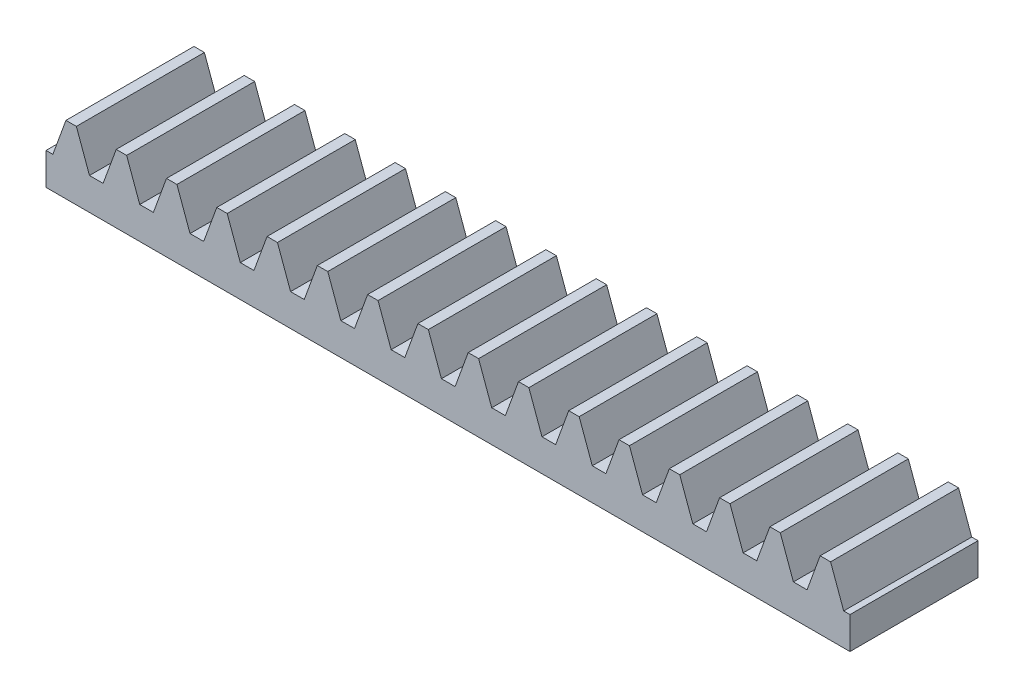
SolidWorks part; units mm, degrees
ref_plane "Front Plane" through (0, 0, 0) normal (0, 0, 1) x (1, 0, 0)
ref_plane "Top Plane" through (0, 0, 0) normal (0, 1, 0) x (1, 0, 0)
ref_plane "Right Plane" through (0, 0, 0) normal (1, 0, 0) x (0, 0, -1)
other "Configuration Table"
sketch "Sketch1" plane through (0, 0, 0) normal (0, 0, 1) x (1, 0, 0)
  line L0 (7.8146, 19.5625) -> (7.6014, 19.5625)
  line L1 (7.6014, 19.5625) -> (7.3966, 20.125)
  line L2 (7.3966, 20.125) -> (7.2339, 20.125)
  line L3 (7.2339, 20.125) -> (7.0292, 19.5625)
  line L4 (7.0292, 19.5625) -> (6.816, 19.5625)
  line L5 (6.816, 19.5625) -> (6.6112, 20.125)
  line L6 (6.6112, 20.125) -> (6.4485, 20.125)
  line L7 (6.4485, 20.125) -> (6.2438, 19.5625)
  line L8 (6.2438, 19.5625) -> (6.0306, 19.5625)
  line L9 (6.0306, 19.5625) -> (5.8258, 20.125)
  line L10 (5.8258, 20.125) -> (5.6631, 20.125)
  line L11 (5.6631, 20.125) -> (5.4584, 19.5625)
  line L12 (5.4584, 19.5625) -> (5.2452, 19.5625)
  line L13 (5.2452, 19.5625) -> (5.0404, 20.125)
  line L14 (5.0404, 20.125) -> (4.8777, 20.125)
  line L15 (4.8777, 20.125) -> (4.673, 19.5625)
  line L16 (4.673, 19.5625) -> (4.4598, 19.5625)
  line L17 (4.4598, 19.5625) -> (4.255, 20.125)
  line L18 (4.255, 20.125) -> (4.0923, 20.125)
  line L19 (4.0923, 20.125) -> (3.8876, 19.5625)
  line L20 (3.8876, 19.5625) -> (3.6744, 19.5625)
  line L21 (3.6744, 19.5625) -> (3.4696, 20.125)
  line L22 (3.4696, 20.125) -> (3.3069, 20.125)
  line L23 (3.3069, 20.125) -> (3.1022, 19.5625)
  line L24 (3.1022, 19.5625) -> (2.889, 19.5625)
  line L25 (2.889, 19.5625) -> (2.6842, 20.125)
  line L26 (2.6842, 20.125) -> (2.5215, 20.125)
  line L27 (2.5215, 20.125) -> (2.3168, 19.5625)
  line L28 (2.3168, 19.5625) -> (2.1036, 19.5625)
  line L29 (2.1036, 19.5625) -> (1.8988, 20.125)
  line L30 (1.8988, 20.125) -> (1.7361, 20.125)
  line L31 (1.7361, 20.125) -> (1.5314, 19.5625)
  line L32 (1.5314, 19.5625) -> (1.3182, 19.5625)
  line L33 (1.3182, 19.5625) -> (1.1134, 20.125)
  line L34 (1.1134, 20.125) -> (0.9507, 20.125)
  line L35 (0.9507, 20.125) -> (0.746, 19.5625)
  line L36 (0.746, 19.5625) -> (0.5328, 19.5625)
  line L37 (0.5328, 19.5625) -> (0.328, 20.125)
  line L38 (0.328, 20.125) -> (0.1653, 20.125)
  line L39 (0.1653, 20.125) -> (-0.0394, 19.5625)
  line L40 (-0.0394, 19.5625) -> (-0.2526, 19.5625)
  line L41 (-0.2526, 19.5625) -> (-0.4574, 20.125)
  line L42 (-0.4574, 20.125) -> (-0.6201, 20.125)
  line L43 (-0.6201, 20.125) -> (-0.8248, 19.5625)
  line L44 (-0.8248, 19.5625) -> (-1.038, 19.5625)
  line L45 (-1.038, 19.5625) -> (-1.2428, 20.125)
  line L46 (-1.2428, 20.125) -> (-1.4055, 20.125)
  line L47 (-1.4055, 20.125) -> (-1.6102, 19.5625)
  line L48 (-1.6102, 19.5625) -> (-1.8234, 19.5625)
  line L49 (-1.8234, 19.5625) -> (-2.0282, 20.125)
  line L50 (-2.0282, 20.125) -> (-2.1909, 20.125)
  line L51 (-2.1909, 20.125) -> (-2.3956, 19.5625)
  line L52 (-2.3956, 19.5625) -> (-2.6088, 19.5625)
  line L53 (-2.6088, 19.5625) -> (-2.8136, 20.125)
  line L54 (-2.8136, 20.125) -> (-2.9763, 20.125)
  line L55 (-2.9763, 20.125) -> (-3.181, 19.5625)
  line L56 (-3.181, 19.5625) -> (-3.3942, 19.5625)
  line L57 (-3.3942, 19.5625) -> (-3.599, 20.125)
  line L58 (-3.599, 20.125) -> (-3.7617, 20.125)
  line L59 (-3.7617, 20.125) -> (-3.9664, 19.5625)
  line L60 (-3.9664, 19.5625) -> (-4.1796, 19.5625)
  line L61 (-4.1796, 19.5625) -> (-4.3844, 20.125)
  line L62 (-4.3844, 20.125) -> (-4.5471, 20.125)
  line L63 (-4.5471, 20.125) -> (-4.7518, 19.5625)
  line L64 (-4.7518, 19.5625) -> (-4.965, 19.5625)
  line L65 (-4.965, 19.5625) -> (-5.1697, 20.125)
  line L66 (-5.1697, 20.125) -> (-5.3325, 20.125)
  line L67 (-5.3325, 20.125) -> (-5.5372, 19.5625)
  line L68 (-5.5372, 19.5625) -> (-5.7504, 19.5625)
  line L69 (-5.7504, 19.5625) -> (-5.9551, 20.125)
  line L70 (-5.9551, 20.125) -> (-6.1179, 20.125)
  line L71 (-6.1179, 20.125) -> (-6.3226, 19.5625)
  line L72 (-6.3226, 19.5625) -> (-6.5358, 19.5625)
  line L73 (-6.5358, 19.5625) -> (-6.7405, 20.125)
  line L74 (-6.7405, 20.125) -> (-6.9033, 20.125)
  line L75 (-6.9033, 20.125) -> (-7.108, 19.5625)
  line L76 (-7.108, 19.5625) -> (-7.3212, 19.5625)
  line L77 (-7.3212, 19.5625) -> (-7.5259, 20.125)
  line L78 (-7.5259, 20.125) -> (-7.6887, 20.125)
  line L79 (-7.6887, 20.125) -> (-7.8934, 19.5625)
  line L80 (-7.8934, 19.5625) -> (-8, 19.5625)
  line L81 (-8, 19.5625) -> (-8, 19.0622)
  line L82 (8, 19.0622) -> (8, 20.072)
  line L83 (8, 20.072) -> (7.8146, 19.5625)
  line L84 (-8, 19.0622) -> (8, 19.0622)
extrude "Boss-Extrude1" add sketch "Sketch1" along normal blind 2
scale "Scale 1" scale about origin uniform scaling yes scale factor 0.7
sketch "Sketch2" plane through (0, 13.3436, 0) normal (0, -1, 0) x (-1, 0, 0)
  line L0 (5.6, -1.4) -> (-5.6, -1.4) construction
  line L1 (-3.1905, -1.4) -> (-5.6, -1.4)
  line L2 (-3.1905, -1.4) -> (-3.1905, 0)
  line L3 (-3.1905, 0) -> (-5.6, 0)
  line L4 (-5.6, -1.4) -> (-5.6, 0)
extrude "Cut-Extrude1" cut sketch "Sketch2" against normal blind 10
